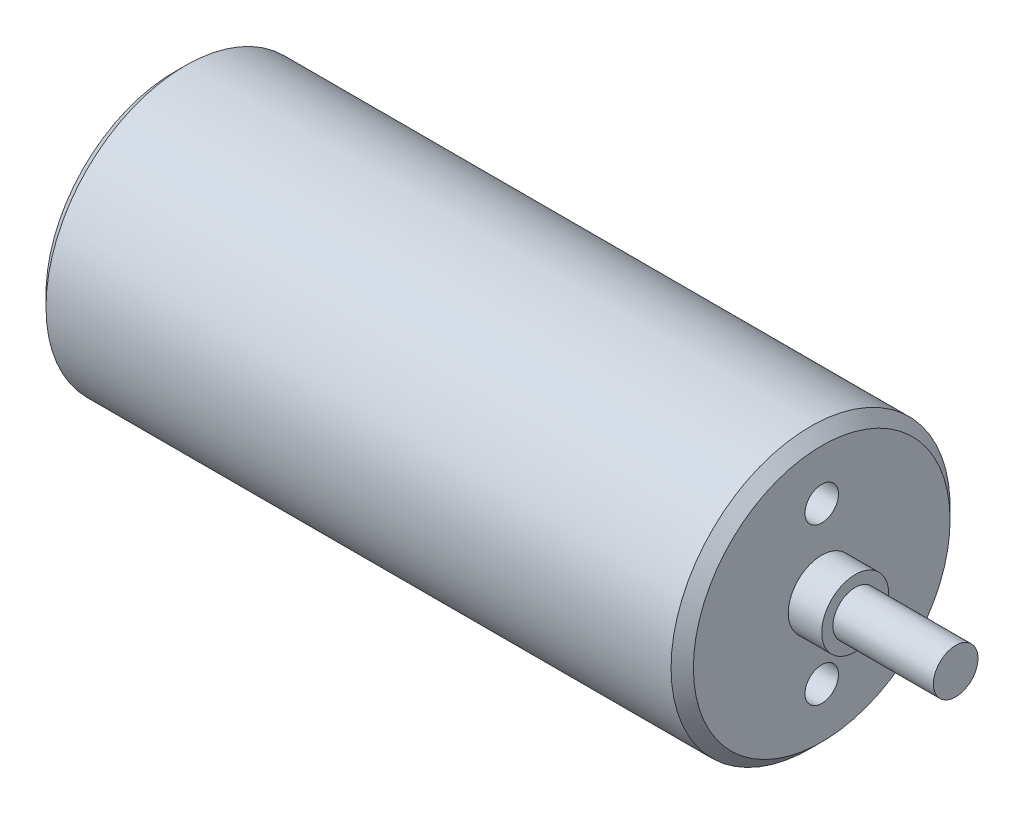
SolidWorks part; units mm, degrees
ref_plane "Front Plane" through (0, 0, 0) normal (0, 0, 1) x (1, 0, 0)
ref_plane "Top Plane" through (0, 0, 0) normal (0, 1, 0) x (1, 0, 0)
ref_plane "Right Plane" through (0, 0, 0) normal (1, 0, 0) x (0, 0, -1)
other "Configuration Table"
sketch "Sketch1" plane through (0, 0, 0) normal (1, 0, 0) x (0, 0, -1)
  circle A0 centre (0, 0) radius 12.5
  dimension "D1" = 25
extrude "Boss-Extrude1" add sketch "Sketch1" along normal blind 58
sketch "Sketch2" plane through (58, 0, 0) normal (1, 0, 0) x (0, 0, -1)
  circle A0 centre (0, 0) radius 3
  dimension "D1" = 6
extrude "Boss-Extrude2" add sketch "Sketch2" along normal blind 3
sketch "Sketch3" plane through (61, 0, 0) normal (1, 0, 0) x (0, 0, -1)
  circle A0 centre (0, 0) radius 2
  dimension "D1" = 4
extrude "Boss-Extrude3" add sketch "Sketch3" along normal blind 9
sketch "Sketch4" plane through (58, 0, 0) normal (1, 0, 0) x (0, 0, -1)
  line L0 (0, 0) -> (-6.3468, 0) construction
  circle A0 centre (0, 0) radius 7 construction
  circle A1 centre (0, 7) radius 1.5
  circle A2 centre (0, -7) radius 1.5
  dimension "D1" = 14
  dimension "D2" = 3
extrude "Cut-Extrude1" cut sketch "Sketch4" against normal blind 6
chamfer "Chamfer1" distance 1 angle 45 1 edges at (58, 0, -12.5)
chamfer "Chamfer2" distance 1 angle 45 1 edges at (0, 0, -12.5)
